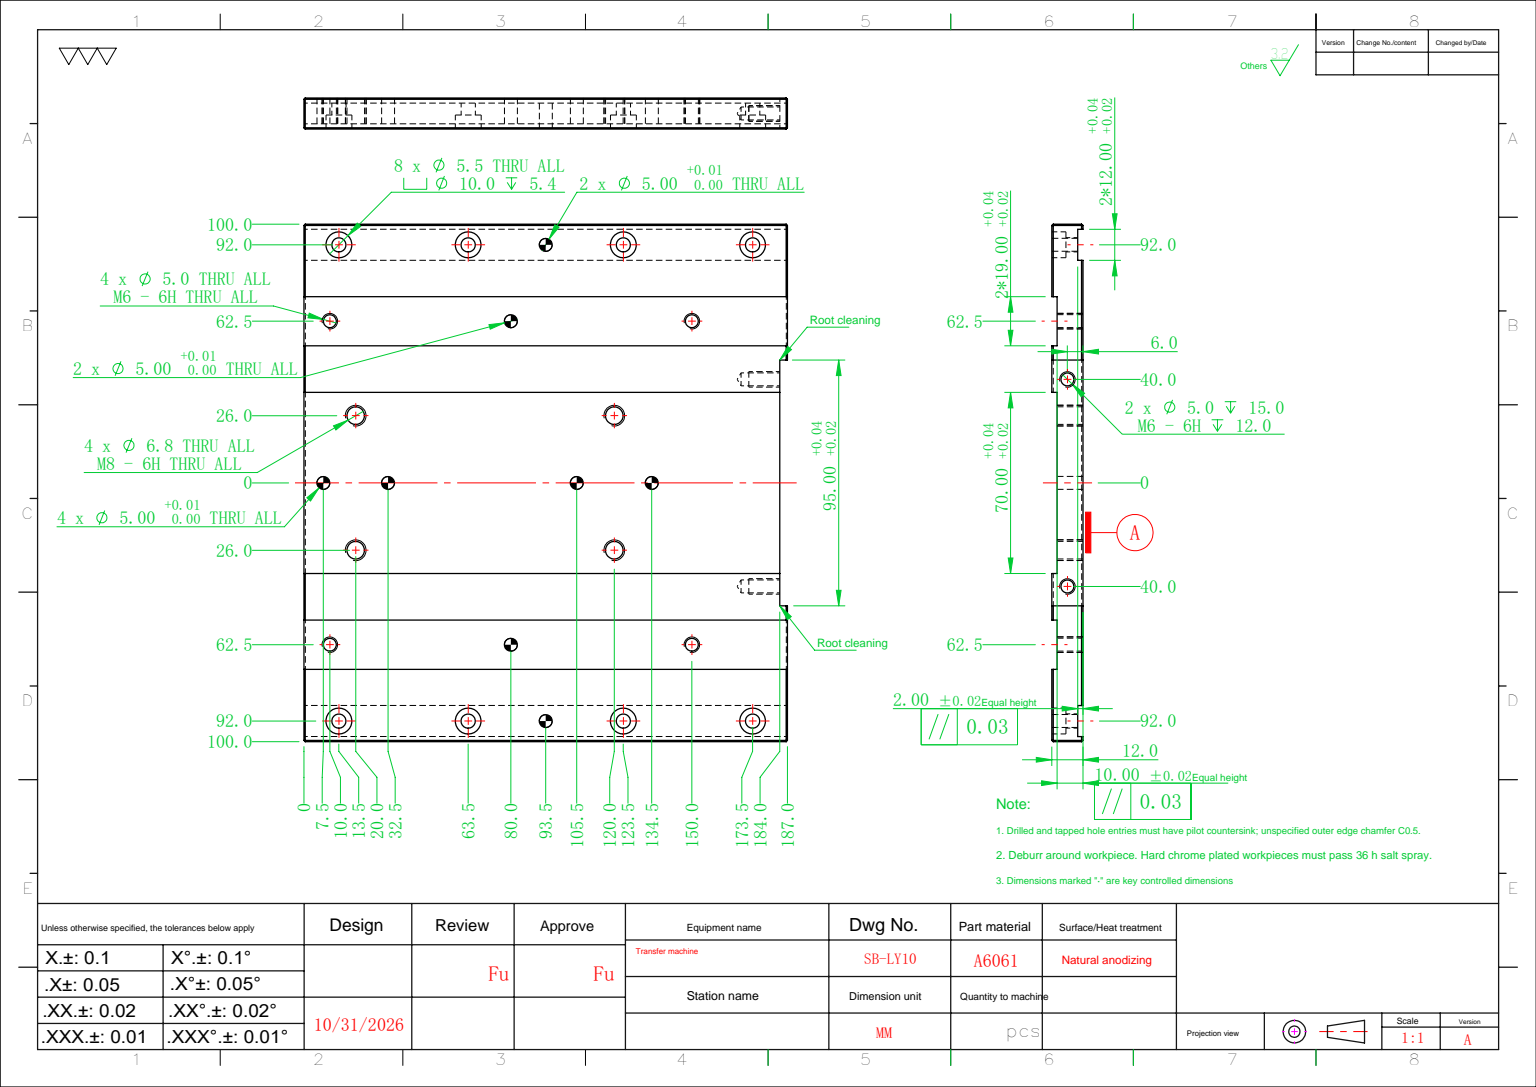
from build123d import *

# Parameters (mm, degrees)
SKETCH_1_W                   = 200
SKETCH_1_H                   = 187
EXTRUDE_1_DEPTH              = 12
SKETCH_4_W                   = 70
SKETCH_4_H                   = 187
CUT_EXTRUDE_3_DEPTH          = 2
SKETCH_5_W                   = 12
SKETCH_5_H                   = 2
CUT_EXTRUDE_4_DEPTH          = 213.398210915
SKETCH_6_W                   = 95
SKETCH_6_H                   = 12
CUT_EXTRUDE_5_DEPTH          = 3
HOLE_WIZARD_M6_1_D           = 5
HOLE_WIZARD_M6_1_DEPTH       = 15
HOLE_WIZARD_M6_1_TIP         = 1.502151548
SKETCH_9_W                   = 19
SKETCH_9_H                   = 187
CUT_EXTRUDE_6_DEPTH          = 2
HOLE_WIZARD_M8_1_D           = 6.8
MM_0_D                       = 5
HOLE_WIZARD_M6_2_D           = 5
MM_1_D                       = 5
HOLE_WIZARD_M5_1_D           = 5.5
HOLE_WIZARD_M5_1_CBORE_D     = 10
HOLE_WIZARD_M5_1_CBORE_DEPTH = 5.4
MM_2_D                       = 5
CHAMFER_1_SIZE               = 0.5


with BuildPart() as part:
    # 草图1 → 凸台-拉伸1 (new body)
    with BuildSketch(Plane.XY):
        Rectangle(SKETCH_1_W, SKETCH_1_H)
    extrude(amount=EXTRUDE_1_DEPTH)

    # 草图4 → 切除-拉伸3 (cut)
    with BuildSketch(Plane(origin=(0, 0, 0), x_dir=(-1, 0, 0), z_dir=(0, 0, -1))):
        Rectangle(SKETCH_4_W, SKETCH_4_H)
    extrude(amount=-CUT_EXTRUDE_3_DEPTH, mode=Mode.SUBTRACT)

    # 草图5 → 切除-拉伸4 (cut, through all)
    with BuildSketch(Plane(origin=(0, 93.5, 0), x_dir=(1, 0, 0), z_dir=(0, 1, 0))):
        with Locations((-92, -11)):
            Rectangle(SKETCH_5_W, SKETCH_5_H)
        with Locations((92, -11)):
            Rectangle(SKETCH_5_W, SKETCH_5_H)
    extrude(amount=-CUT_EXTRUDE_4_DEPTH, mode=Mode.SUBTRACT)

    # 草图6 → 切除-拉伸5 (cut)
    with BuildSketch(Plane(origin=(0, 93.5, 0), x_dir=(1, 0, 0), z_dir=(0, 1, 0))):
        with Locations((0, -6)):
            Rectangle(SKETCH_6_W, SKETCH_6_H)
    extrude(amount=-CUT_EXTRUDE_5_DEPTH, mode=Mode.SUBTRACT)

    # M6 螺纹孔1
    with Locations(Plane(origin=(0, 90.5, 0), x_dir=(1, 0, 0), z_dir=(0, 1, 0))):
        with Locations((-40, -6), (40, -6)):
            Hole(HOLE_WIZARD_M6_1_D / 2, depth=HOLE_WIZARD_M6_1_DEPTH)
            with Locations((0, 0, -(HOLE_WIZARD_M6_1_DEPTH + HOLE_WIZARD_M6_1_TIP / 2))):  # 118° drill point
                Cone(0, HOLE_WIZARD_M6_1_D / 2, HOLE_WIZARD_M6_1_TIP, mode=Mode.SUBTRACT)

    # 草图9 → 切除-拉伸6 (cut)
    with BuildSketch(Plane(origin=(0, 0, 0), x_dir=(-1, 0, 0), z_dir=(0, 0, -1))):
        with Locations((-62.5, 0)):
            Rectangle(SKETCH_9_W, SKETCH_9_H)
        with Locations((62.5, 0)):
            Rectangle(SKETCH_9_W, SKETCH_9_H)
    extrude(amount=-CUT_EXTRUDE_6_DEPTH, mode=Mode.SUBTRACT)

    # M8 螺纹孔1 (through all)
    with Locations(Plane(origin=(0, 0, 0), x_dir=(-1, 0, 0), z_dir=(0, 0, -1))):
        with Locations((26, -73.5), (-26, -73.5), (26, 26.5), (-26, 26.5)):
            Hole(HOLE_WIZARD_M8_1_D / 2)

    # 大小mm 暗销孔0 (through all)
    with Locations(Plane(origin=(0, 0, 2), x_dir=(-1, 0, 0), z_dir=(0, 0, -1))):
        with Locations((0, -86), (0, -61), (0, 12), (0, 41)):
            Hole(MM_0_D / 2)

    # M6 螺纹孔2 (through all)
    with Locations(Plane(origin=(0, 0, 2), x_dir=(-1, 0, 0), z_dir=(0, 0, -1))):
        with Locations((62.5, -83.5), (62.5, 56.5), (-62.5, 56.5), (-62.5, -83.5)):
            Hole(HOLE_WIZARD_M6_2_D / 2)

    # 大小mm 暗销孔1 (through all)
    with Locations(Plane(origin=(0, 0, 2), x_dir=(-1, 0, 0), z_dir=(0, 0, -1))):
        with Locations((-62.5, -13.5), (62.5, -13.5)):
            Hole(MM_1_D / 2)

    # M5 六角凹头螺钉的柱形沉头孔1 (through all)
    with Locations(Plane(origin=(0, 0, 0), x_dir=(-1, 0, 0), z_dir=(0, 0, -1))):
        with Locations((-92, 80), (-92, -80), (-92, 30), (-92, -30), (92, -30), (92, 30), (92, -80), (92, 80)):
            CounterBoreHole(HOLE_WIZARD_M5_1_D / 2, HOLE_WIZARD_M5_1_CBORE_D / 2, HOLE_WIZARD_M5_1_CBORE_DEPTH)

    # 大小mm 暗销孔2 (through all)
    with Locations(Plane(origin=(0, 0, 0), x_dir=(-1, 0, 0), z_dir=(0, 0, -1))):
        with Locations((92, 0), (-92, 0)):
            Hole(MM_2_D / 2)

    # 倒角1
    chamfer_1_edges = [part.edges().sort_by_distance(p)[0] for p in [
        (-100, 0, 12),
        (50.25, 93.5, 0),
        (-99, -93.5, 12),
        (44, -93.5, 0),
        (66.75, 93.5, 12),
        (-99, 93.5, 12),
        (0, -93.5, 12),
        (99, -93.5, 12),
        (100, 0, 12),
        (-86, -93.5, 0),
        (-100, 0, 0),
        (86, 93.5, 0),
        (100, 0, 0),
        (-50.25, 93.5, 0),
        (-66.75, 93.5, 12),
        (99, 93.5, 12),
        (100, -93.5, 6),
        (-100, -93.5, 6),
        (-100, 93.5, 6),
        (100, 93.5, 6),
        (-44, -93.5, 0),
        (-86, 93.5, 0),
        (86, -93.5, 0),
    ]]
    chamfer(chamfer_1_edges, length=CHAMFER_1_SIZE)


solid = part.part
